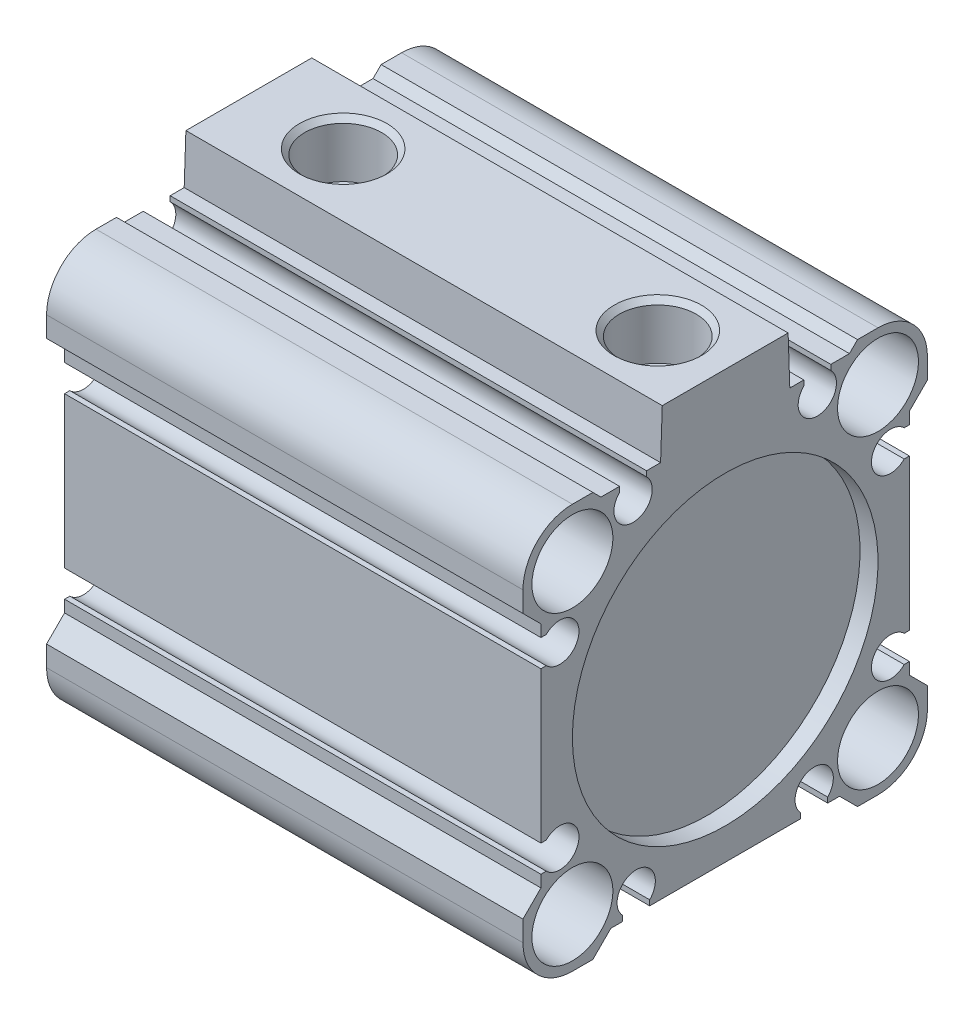
from build123d import *

# Parameters (mm, degrees)
BOSS_EXTRUDE1_DEPTH  = 53
SKETCH2_W            = 2
SKETCH2_H            = 17
CUT_EXTRUDE1_START   = 5
SKETCH3_R            = 17
SKETCH3_R_2          = 10.5
CUT_EXTRUDE1_DEPTH   = 5
LPATTERN1_COUNT      = 2
LPATTERN1_PITCH      = 34
LPATTERN1_COUNT_DIR2 = 2
LPATTERN1_PITCH_DIR2 = 34


with BuildPart() as part:
    # Sketch1 → Boss-Extrude1 (new body)
    with BuildSketch(Plane(origin=(0, 0, 0), x_dir=(0, 0, -1), z_dir=(1, 0, 0))):
        with BuildLine():
            Line((-22.5, 17), (-22.5, 14.721825407))
            Line((-22.5, 14.721825407), (-20.5, 12.721825407))
            Line((-20.5, 12.721825407), (-20.5, 11.4))
            Line((-20.5, 11.4), (-19.912249979, 11.4))
            ThreePointArc((-19.912249979, 11.4), (-16.27, 9.9), (-19.912249979, 8.4))
            Line((-19.912249979, 8.4), (-20.5, 8.4))
            Line((-20.5, 8.4), (-20.5, -8.4))
            Line((-20.5, -8.4), (-19.912249979, -8.4))
            ThreePointArc((-19.912249979, -8.4), (-16.27, -9.9), (-19.912249979, -11.4))
            Line((-19.912249979, -11.4), (-20.5, -11.4))
            Line((-20.5, -11.4), (-20.5, -12.721825407))
            Line((-20.5, -12.721825407), (-22.5, -14.721825407))
            Line((-22.5, -14.721825407), (-22.5, -17))
            ThreePointArc((-22.5, -17), (-20.889087297, -20.889087297), (-17, -22.5))
            Line((-17, -22.5), (-14.721825407, -22.5))
            Line((-14.721825407, -22.5), (-12.721825407, -20.5))
            Line((-12.721825407, -20.5), (-11.4, -20.5))
            Line((-11.4, -20.5), (-11.4, -19.912249979))
            ThreePointArc((-11.4, -19.912249979), (-9.9, -16.27), (-8.4, -19.912249979))
            Line((-8.4, -19.912249979), (-8.4, -20.5))
            Line((-8.4, -20.5), (8.4, -20.5))
            Line((8.4, -20.5), (8.4, -19.912249979))
            ThreePointArc((8.4, -19.912249979), (9.9, -16.27), (11.4, -19.912249979))
            Line((11.4, -19.912249979), (11.4, -20.5))
            Line((11.4, -20.5), (12.721825407, -20.5))
            Line((12.721825407, -20.5), (14.721825407, -22.5))
            Line((14.721825407, -22.5), (17, -22.5))
            ThreePointArc((17, -22.5), (20.889087297, -20.889087297), (22.5, -17))
            Line((22.5, -17), (22.5, -14.721825407))
            Line((22.5, -14.721825407), (20.5, -12.721825407))
            Line((20.5, -12.721825407), (20.5, -11.4))
            Line((20.5, -11.4), (19.912249979, -11.4))
            ThreePointArc((19.912249979, -11.4), (16.27, -9.9), (19.912249979, -8.4))
            Line((19.912249979, -8.4), (20.5, -8.4))
            Line((20.5, -8.4), (20.5, 8.4))
            Line((20.5, 8.4), (19.912249979, 8.4))
            ThreePointArc((19.912249979, 8.4), (16.27, 9.9), (19.912249979, 11.4))
            Line((19.912249979, 11.4), (20.5, 11.4))
            Line((20.5, 11.4), (20.5, 12.721825407))
            Line((20.5, 12.721825407), (22.5, 14.721825407))
            Line((22.5, 14.721825407), (22.5, 17))
            ThreePointArc((22.5, 17), (20.889087297, 20.889087297), (17, 22.5))
            Line((17, 22.5), (14.721825407, 22.5))
            Line((14.721825407, 22.5), (13.821825407, 21.6))
            Line((13.821825407, 21.6), (11.75, 21.6))
            Line((11.75, 21.6), (11.75, 21.012249979))
            ThreePointArc((11.75, 21.012249979), (10.25, 17.37), (8.75, 21.012249979))
            Line((8.75, 21.012249979), (8.75, 21.6))
            Line((8.75, 21.6), (7.188572155, 21.6))
            Line((7.188572155, 21.6), (7, 27))
            Line((7, 27), (-7, 27))
            Line((-7, 27), (-7.188572155, 21.6))
            Line((-7.188572155, 21.6), (-8.75, 21.6))
            Line((-8.75, 21.6), (-8.75, 21.012249979))
            ThreePointArc((-8.75, 21.012249979), (-10.25, 17.37), (-11.75, 21.012249979))
            Line((-11.75, 21.012249979), (-11.75, 21.6))
            Line((-11.75, 21.6), (-13.821825407, 21.6))
            Line((-13.821825407, 21.6), (-14.721825407, 22.5))
            Line((-14.721825407, 22.5), (-17, 22.5))
            ThreePointArc((-17, 22.5), (-20.889087297, 20.889087297), (-22.5, 17))
        make_face()
    extrude(amount=BOSS_EXTRUDE1_DEPTH)

    # Sketch2 → Cut-Revolve1 (revolve, cut)
    with BuildSketch(Plane.XY, mode=Mode.PRIVATE) as cut_revolve1_sk:
        with Locations((52, 8.5)):
            Rectangle(SKETCH2_W, SKETCH2_H)
    revolve(cut_revolve1_sk.sketch.rotate(Axis((53, 0, 0), (-1, 0, 0)), 270), axis=Axis((53, 0, 0), (-1, 0, 0)), mode=Mode.SUBTRACT)

    # Sketch3 → Cut-Extrude1 (cut)
    with BuildSketch(Plane(origin=(0, 0, 0), x_dir=(0, 0, -1), z_dir=(1, 0, 0)).offset(CUT_EXTRUDE1_START)):
        with Locations(Location((0, 0, 0), (0, 0, 180))):
            Circle(SKETCH3_R)
        Circle(SKETCH3_R_2, mode=Mode.SUBTRACT)
    extrude(amount=-CUT_EXTRUDE1_DEPTH, mode=Mode.SUBTRACT)

    # Sketch4 → Cut-Revolve2 (revolve, cut)
    with BuildSketch(Plane.XY, mode=Mode.PRIVATE) as cut_revolve2_sk:
        Polygon((0, 0), (0, 8), (10, 8), (10, 16), (35, 16), (35, 0), align=None)
    revolve(cut_revolve2_sk.sketch.rotate(Axis((35, 0, 0), (-1, 0, 0)), 270), axis=Axis((35, 0, 0), (-1, 0, 0)), mode=Mode.SUBTRACT)

    # Sketch5 → Cut-Revolve3 (revolve, cut)
    with BuildSketch(Plane.XY, mode=Mode.PRIVATE) as cut_revolve3_sk:
        Polygon((10.5, 27), (15.364, 27), (14.783, 26.419), (14.783, 20.8), (10.5, 20.8), align=None)
    revolve(cut_revolve3_sk.sketch.rotate(Axis((10.5, 20.8, 0), (0, 1, 0)), 180), axis=Axis((10.5, 20.8, 0), (0, 1, 0)), mode=Mode.SUBTRACT)

    # Sketch6 → Cut-Revolve4 (revolve, cut)
    with BuildSketch(Plane.XY, mode=Mode.PRIVATE) as cut_revolve4_sk:
        Polygon((45.5, 27), (50.364, 27), (49.783, 26.419), (49.783, 20.8), (45.5, 20.8), align=None)
    revolve(cut_revolve4_sk.sketch.rotate(Axis((45.5, 20.8, 0), (0, 1, 0)), 180), axis=Axis((45.5, 20.8, 0), (0, 1, 0)), mode=Mode.SUBTRACT)

    # Sketch7 → Cut-Revolve5 (revolve, cut)
    with BuildSketch(Plane.XY.offset(17), mode=Mode.PRIVATE) as cut_revolve5_sk:
        Polygon((0, 17), (0, 21.5), (7, 21.5), (7, 19.75), (46, 19.75), (46, 21.5), (53, 21.5), (53, 17), align=None)
    cut_revolve5 = revolve(cut_revolve5_sk.sketch.rotate(Axis((53, 17, 17), (-1, 0, 0)), 270), axis=Axis((53, 17, 17), (-1, 0, 0)), mode=Mode.SUBTRACT)

    # LPattern1: Cut-Revolve5 2 × 2
    with Locations(*[(0, -j * LPATTERN1_PITCH_DIR2, -i * LPATTERN1_PITCH) for i in range(LPATTERN1_COUNT) for j in range(LPATTERN1_COUNT_DIR2) if (i, j) != (0, 0)]):
        add(cut_revolve5, mode=Mode.SUBTRACT)


solid = part.part
